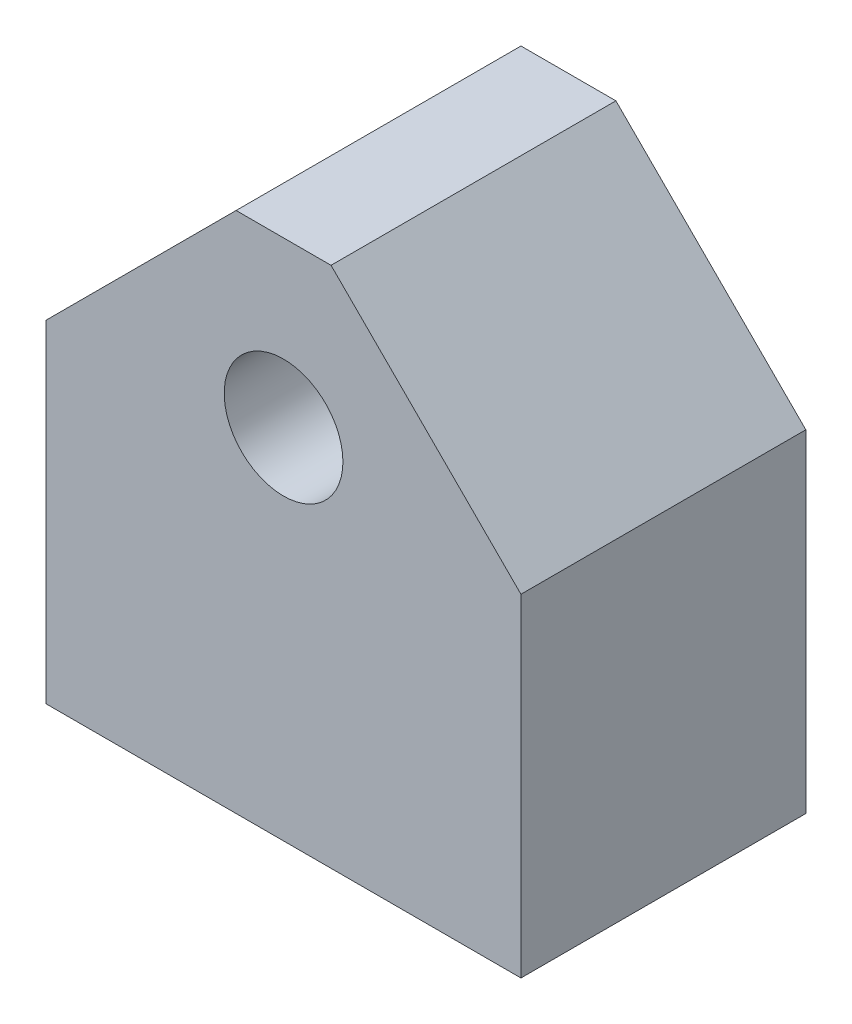
SolidWorks part; units mm, degrees
material "1023 碳钢板 (SS)"
ref_plane "前视基准面" through (0, 0, 0) normal (0, 0, 1) x (1, 0, 0)
ref_plane "上视基准面" through (0, 0, 0) normal (0, 1, 0) x (1, 0, 0)
ref_plane "右视基准面" through (0, 0, 0) normal (1, 0, 0) x (0, 0, -1)
sketch "草图1" plane through (0, 0, 0) normal (0, 0, 1) x (1, 0, 0)
  line L1 (-25, 27.5) -> (25, 27.5)
  line L2 (-25, 27.5) -> (-25, -27.5)
  line L3 (-25, -27.5) -> (25, -27.5)
  line L4 (25, 27.5) -> (25, -27.5)
  line L5 (-25, 27.5) -> (25, -27.5) construction
  line L6 (-25, -27.5) -> (25, 27.5) construction
  point P0 (0, 0)
  dimension "D1" = 50
  dimension "D2" = 55
extrude "凸台-拉伸1" add sketch "草图1" along normal blind 30
chamfer "倒角1" distance 20 angle 45 2 edges at (25, 27.5, 15) (-25, 27.5, 15)
sketch "草图2" plane through (0, -27.5, 0) normal (0, -1, 0) x (1, 0, 0)
  line L0 (-25, 30) -> (25, 30) construction
  line L1 (-25, 30) -> (-25, 0) construction
  circle A0 centre (-15, 15) radius 5 construction
  circle A1 centre (15, 15) radius 5 construction
  dimension "D5" = 10
  dimension "D1" = 15
  dimension "D2" = 15
  dimension "D3" = 30
  dimension "D4" = 10
hole_wizard "M10 螺纹孔1" positions "草图3" profile "草图4" tap size "M10" standard "GB"
sketch "草图3" plane through (0, -27.5, 0) normal (0, -1, 0) x (-1, 0, 0)
  point P0 (15, -15)
  point P3 (-15, -15)
sketch "草图4" plane through (-15, -27.5, 15) normal (1, 0, 0) x (0, 0, -1)
  line L0 (0, 0) -> (0, 27.0537)
  line L1 (0, 27.0537) -> (4.25, 24.5)
  line L2 (4.25, 24.5) -> (4.25, 0)
  line L5 (4.25, 0) -> (0, 0)
  line L10 (0, 27.0537) -> (-4.25, 24.5) construction
  line L11 (0, -6.35) -> (0, 107.95) construction
  dimension "螺纹孔钻头直径" = 8.5
  dimension "螺纹孔钻头深度" = 24.5
  dimension "导头角度" = 118
cosmetic thread "孔螺蚊线1" parameters "D1"=20, "D2"=10
cosmetic thread "孔螺蚊线2" parameters "D1"=20, "D2"=10
sketch "草图5" plane through (0, 0, 30) normal (0, 0, 1) x (1, 0, 0)
  line L0 (-25, -27.5) -> (25, -27.5) construction
  circle A0 centre (0, 10.2) radius 6.25
  dimension "D1" = 12.5
  dimension "D2" = 37.7
extrude "切除-拉伸1" cut sketch "草图5" against normal blind 30
